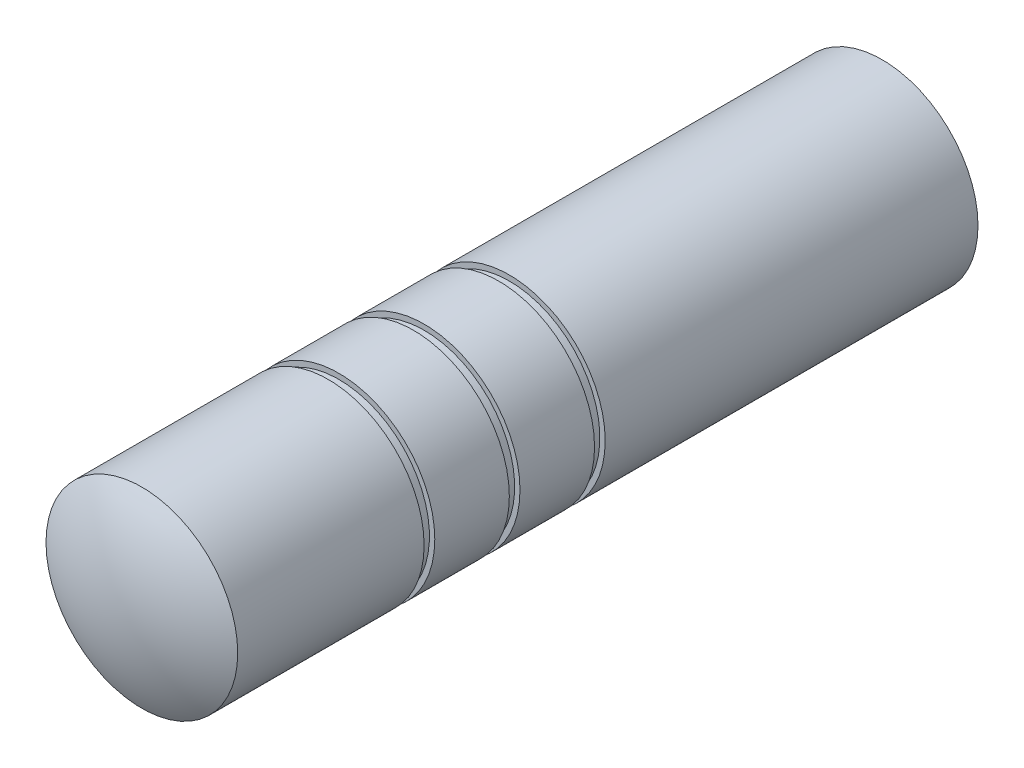
from build123d import *

# Parameters (mm, degrees)
SKETCH1_R                   = 9
BOSS_EXTRUDE1_DEPTH         = 69.5
SKETCH2_R                   = 7
CUT_EXTRUDE1_DEPTH          = 32
CUT_EXTRUDE3_START          = -35
SKETCH3_R                   = 9
SKETCH3_R_2                 = 8.5
CUT_EXTRUDE3_DEPTH          = 1
CUT_EXTRUDE4_START          = -7
SKETCH4_R                   = 9
SKETCH4_R_2                 = 8.5
CUT_EXTRUDE4_DEPTH          = 1
CUT_EXTRUDE5_START          = -7
SKETCH5_R                   = 9
SKETCH5_R_2                 = 8.5
CUT_EXTRUDE5_DEPTH          = 1
M5_TAPPED_HOLE1_D           = 4.2
M5_TAPPED_HOLE1_DEPTH       = 8.7381927
M5_TAPPED_HOLE1_CSINK_D     = 5.05
M5_TAPPED_HOLE1_CSINK_ANGLE = 90
M5_TAPPED_HOLE1_TIP         = 1.2618073


with BuildPart() as part:
    # Sketch1 → Boss-Extrude1 (new body)
    with BuildSketch(Plane.XY):
        Circle(SKETCH1_R)
    extrude(amount=BOSS_EXTRUDE1_DEPTH)

    # Sketch2 → Cut-Extrude1 (cut)
    with BuildSketch(Plane(origin=(0, 0, 0), x_dir=(-1, 0, 0), z_dir=(0, 0, -1))):
        Circle(SKETCH2_R)
    extrude(amount=-CUT_EXTRUDE1_DEPTH, mode=Mode.SUBTRACT)

    # Sketch3 → Cut-Extrude3 (cut)
    with BuildSketch(Plane(origin=(0, 0, 0), x_dir=(-1, 0, 0), z_dir=(0, 0, -1)).offset(CUT_EXTRUDE3_START)):
        Circle(SKETCH3_R)
        Circle(SKETCH3_R_2, mode=Mode.SUBTRACT)
    extrude(amount=-CUT_EXTRUDE3_DEPTH, mode=Mode.SUBTRACT)

    # Sketch4 → Cut-Extrude4 (cut)
    with BuildSketch(Plane(origin=(0, 0, 36), x_dir=(-1, 0, 0), z_dir=(0, 0, -1)).offset(CUT_EXTRUDE4_START)):
        Circle(SKETCH4_R)
        Circle(SKETCH4_R_2, mode=Mode.SUBTRACT)
    extrude(amount=-CUT_EXTRUDE4_DEPTH, mode=Mode.SUBTRACT)

    # Sketch5 → Cut-Extrude5 (cut)
    with BuildSketch(Plane(origin=(0, 0, 44), x_dir=(-1, 0, 0), z_dir=(0, 0, -1)).offset(CUT_EXTRUDE5_START)):
        Circle(SKETCH5_R)
        Circle(SKETCH5_R_2, mode=Mode.SUBTRACT)
    extrude(amount=-CUT_EXTRUDE5_DEPTH, mode=Mode.SUBTRACT)

    # Sketch6 → Revolve1 (revolve)
    with BuildSketch(Plane(origin=(0, 0, 0), x_dir=(1, 0, 0), z_dir=(0, 1, 0))):
        with BuildLine():
            Line((0, -69.5), (0, -71.99166898))
            ThreePointArc((0, -71.99166898), (-4.669272275, -71.357252173), (-9, -69.5))
            Line((-9, -69.5), (0, -69.5))
        make_face()
    revolve(axis=Axis((0, 0, 0), (0, 0, 1)))

    # M5 Tapped Hole1
    with Locations(Plane(origin=(0, 0, 32), x_dir=(-1, 0, 0), z_dir=(0, 0, -1))):
        with Locations((0, 0)):
            CounterSinkHole(M5_TAPPED_HOLE1_D / 2, M5_TAPPED_HOLE1_CSINK_D / 2, depth=M5_TAPPED_HOLE1_DEPTH, counter_sink_angle=M5_TAPPED_HOLE1_CSINK_ANGLE)
            with Locations((0, 0, -(M5_TAPPED_HOLE1_DEPTH + M5_TAPPED_HOLE1_TIP / 2))):  # 118° drill point
                Cone(0, M5_TAPPED_HOLE1_D / 2, M5_TAPPED_HOLE1_TIP, mode=Mode.SUBTRACT)


solid = part.part
